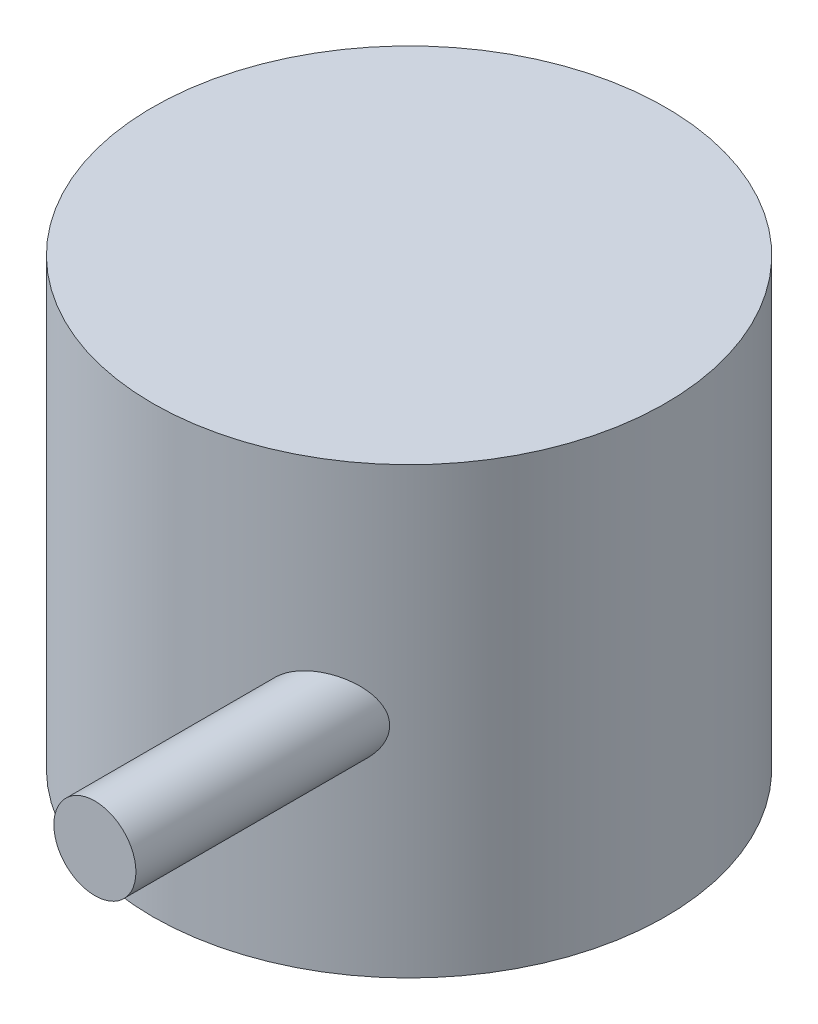
from build123d import *

# Parameters (mm, degrees)
SKETCH1_R           = 37.5
BOSS_EXTRUDE1_DEPTH = 65
SKETCH2_R           = 6
BOSS_EXTRUDE2_DEPTH = 65


with BuildPart() as part:
    # Sketch1 → Boss-Extrude1 (new body)
    with BuildSketch(Plane(origin=(0, 0, 0), x_dir=(1, 0, 0), z_dir=(0, 1, 0))):
        with Locations(Location((0, 0, 0), (0, 0, 270))):
            Circle(SKETCH1_R)
    extrude(amount=BOSS_EXTRUDE1_DEPTH)

    # Sketch2 → Boss-Extrude2 (add)
    with BuildSketch(Plane.XY):
        with Locations(Location((19.06, 31.933431832, 0), (0, 0, 180))):
            Circle(SKETCH2_R)
    extrude(amount=BOSS_EXTRUDE2_DEPTH)


solid = part.part
